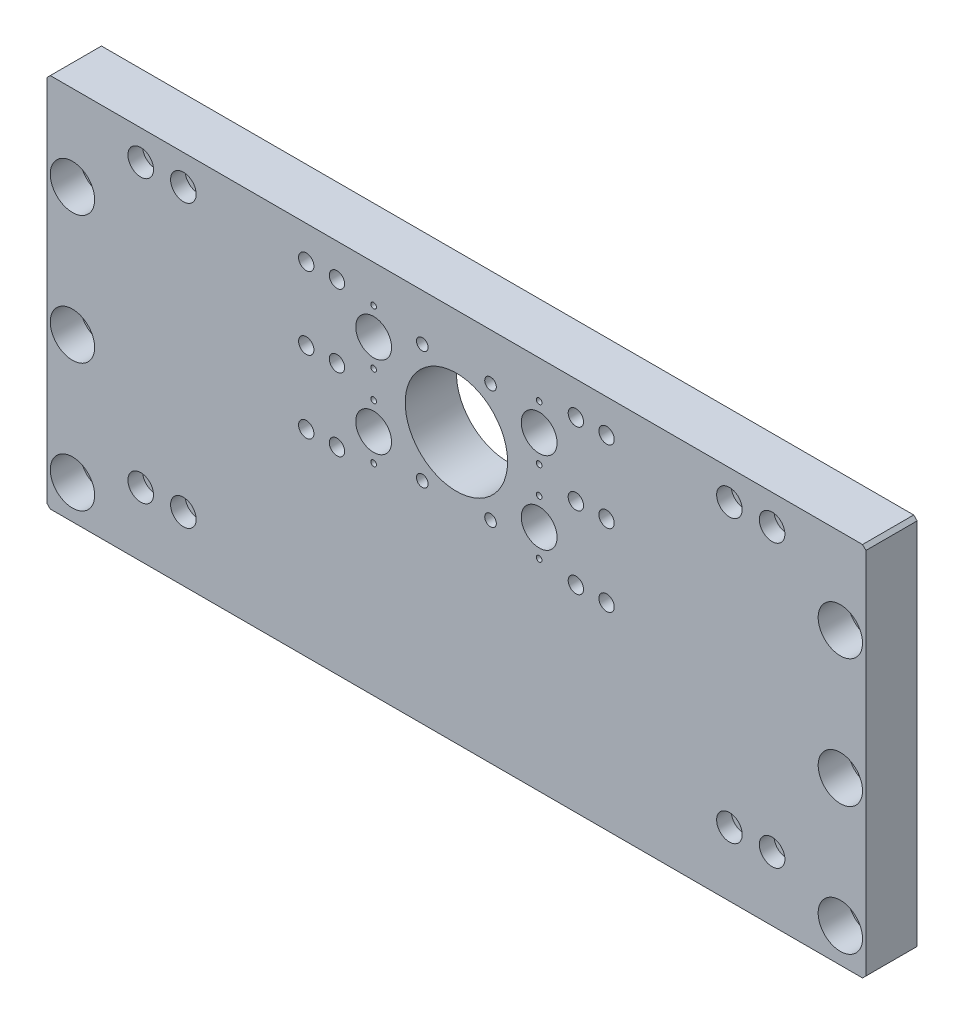
from build123d import *

# Parameters (mm, degrees)
SKETCH1_W                                            = 480
SKETCH1_H                                            = 220
BOSS_EXTRUDE1_DEPTH                                  = 15
HOLE_SIZE_PER_SOCKET_HEAD_CAP_SCREW_TYPE_D           = 17.5
HOLE_SIZE_PER_SOCKET_HEAD_CAP_SCREW_TYPE_CBORE_D     = 26
HOLE_SIZE_PER_SOCKET_HEAD_CAP_SCREW_TYPE_CBORE_DEPTH = 17.5
CHAMFER1_SIZE                                        = 2
SKETCH4_R                                            = 30
CUT_EXTRUDE1_DEPTH                                   = 266.706605112
M8_TAPPED_HOLE1_D                                    = 6.8
M8_TAPPED_HOLE1_DEPTH                                = 19.75
M8_TAPPED_HOLE1_TIP                                  = 2.042926105
HOLE_WIZARD_2_D                                      = 9
HOLE_WIZARD_2_CBORE_D                                = 15
HOLE_WIZARD_2_CBORE_DEPTH                            = 9
SKETCH9_R                                            = 10.5
CUT_EXTRUDE2_DEPTH                                   = 266.706605112
M4_TAPPED_HOLE1_AT_2_COUNT                           = 2
M4_TAPPED_HOLE1_AT_2_PITCH                           = 32
M4_TAPPED_HOLE1_AT_3_COUNT                           = 2
M4_TAPPED_HOLE1_AT_3_PITCH                           = 48
M4_TAPPED_HOLE1_AT_4_COUNT                           = 2
M4_TAPPED_HOLE1_AT_4_PITCH                           = 80
CBORE_FOR_M8_HEX_SOCKET_HEAD_CAP_SCREW1_D            = 9
CBORE_FOR_M8_HEX_SOCKET_HEAD_CAP_SCREW1_CBORE_D      = 15
CBORE_FOR_M8_HEX_SOCKET_HEAD_CAP_SCREW1_CBORE_DEPTH  = 8.6


with BuildPart() as part:
    # Sketch1 → Boss-Extrude1 (new, symmetric)
    with BuildSketch(Plane.XY):
        Rectangle(SKETCH1_W, SKETCH1_H)
    extrude(amount=BOSS_EXTRUDE1_DEPTH, both=True)

    # Hole size per socket head cap screw type2 (through all)
    with Locations(Plane.XY.offset(15)):
        with Locations((-225, 60), (225, 60), (225, -90), (-225, -90), (-225, -15), (225, -15)):
            CounterBoreHole(HOLE_SIZE_PER_SOCKET_HEAD_CAP_SCREW_TYPE_D / 2, HOLE_SIZE_PER_SOCKET_HEAD_CAP_SCREW_TYPE_CBORE_D / 2, HOLE_SIZE_PER_SOCKET_HEAD_CAP_SCREW_TYPE_CBORE_DEPTH)

    # Chamfer1
    chamfer1_edges = [part.edges().sort_by_distance(p)[0] for p in [
        (240, -110, 0),
        (-240, -110, 0),
        (-240, 110, 0),
        (240, 110, 0),
    ]]
    chamfer(chamfer1_edges, length=CHAMFER1_SIZE)

    # Sketch4 → Cut-Extrude1 (cut, through all)
    with BuildSketch(Plane.XY.offset(15)):
        with Locations((0, 48)):
            Circle(SKETCH4_R)
    extrude(amount=-CUT_EXTRUDE1_DEPTH, mode=Mode.SUBTRACT)

    # M8 Tapped Hole1
    with Locations(Plane.XY.offset(15)):
        with Locations((-20, 82.641016151), (20, 82.641016151), (-20, 13.358983849), (20, 13.358983849)):
            Hole(M8_TAPPED_HOLE1_D / 2, depth=M8_TAPPED_HOLE1_DEPTH)
            with Locations((0, 0, -(M8_TAPPED_HOLE1_DEPTH + M8_TAPPED_HOLE1_TIP / 2))):  # 118° drill point
                Cone(0, M8_TAPPED_HOLE1_D / 2, M8_TAPPED_HOLE1_TIP, mode=Mode.SUBTRACT)

    # 打孔尺寸根据内六角圆柱头螺钉的类型2 (through all)
    with Locations(Plane(origin=(0, 0, -15), x_dir=(-1, 0, 0), z_dir=(0, 0, -1))):
        with Locations((-88, 90.5), (-70, 90.5), (-70, 48), (-88, 48), (-88, 5.5), (-70, 5.5), (70, 90.5), (88, 90.5), (70, 48), (88, 48), (70, 5.5), (88, 5.5)):
            CounterBoreHole(HOLE_WIZARD_2_D / 2, HOLE_WIZARD_2_CBORE_D / 2, HOLE_WIZARD_2_CBORE_DEPTH)

    # Sketch9 → Cut-Extrude2 (cut, through all)
    with BuildSketch(Plane.XY.offset(15)):
        with Locations((-48.5, 72)):
            Circle(SKETCH9_R)
        with Locations((-48.5, 24)):
            Circle(SKETCH9_R)
        with Locations((48.5, 24)):
            Circle(SKETCH9_R)
        with Locations((48.5, 72)):
            Circle(SKETCH9_R)
    extrude(amount=-CUT_EXTRUDE2_DEPTH, mode=Mode.SUBTRACT)

    # Sketch10 → M4 Tapped Hole1 (revolve, cut)
    with BuildSketch(Plane(origin=(48.5, 88, 15), x_dir=(0, -1, 0), z_dir=(1, 0, 0))):
        Polygon((0, 0), (0, 11.091420021), (1.65, 10.1), (1.65, 0), align=None)
    m4_tapped_hole1 = revolve(axis=Axis((48.5, 88, 21.35), (0, 0, -1)), mode=Mode.SUBTRACT)

    # M4 Tapped Hole1 at 2: M4 Tapped Hole1 ×2
    with Locations(*[(0, -i * M4_TAPPED_HOLE1_AT_2_PITCH, 0) for i in range(1, M4_TAPPED_HOLE1_AT_2_COUNT)]):
        add(m4_tapped_hole1, mode=Mode.SUBTRACT)

    # M4 Tapped Hole1 at 3: M4 Tapped Hole1 ×2
    with Locations(*[(0, -i * M4_TAPPED_HOLE1_AT_3_PITCH, 0) for i in range(1, M4_TAPPED_HOLE1_AT_3_COUNT)]):
        add(m4_tapped_hole1, mode=Mode.SUBTRACT)

    # M4 Tapped Hole1 at 4: M4 Tapped Hole1 ×2
    with Locations(*[(0, -i * M4_TAPPED_HOLE1_AT_4_PITCH, 0) for i in range(1, M4_TAPPED_HOLE1_AT_4_COUNT)]):
        add(m4_tapped_hole1, mode=Mode.SUBTRACT)

    # Mirror1: M4 Tapped Hole1 across plane
    add(m4_tapped_hole1.mirror(Plane(origin=(0, 0, 0), x_dir=(0, 0, 1), z_dir=(1, 0, 0))), mode=Mode.SUBTRACT)

    # Mirror1 copy 1 sketch → Mirror1 copy 1 (revolve, cut)
    with BuildSketch(Plane(origin=(-48.5, 56, 15), x_dir=(0, -1, 0), z_dir=(-1, 0, 0))):
        Polygon((0, 0), (0, -11.091420021), (1.65, -10.1), (1.65, 0), align=None)
    revolve(axis=Axis((-48.5, 56, 21.35), (0, 0, 1)), mode=Mode.SUBTRACT)

    # Mirror1 copy 2 sketch → Mirror1 copy 2 (revolve, cut)
    with BuildSketch(Plane(origin=(-48.5, 40, 15), x_dir=(0, -1, 0), z_dir=(-1, 0, 0))):
        Polygon((0, 0), (0, -11.091420021), (1.65, -10.1), (1.65, 0), align=None)
    revolve(axis=Axis((-48.5, 40, 21.35), (0, 0, 1)), mode=Mode.SUBTRACT)

    # Mirror1 copy 3 sketch → Mirror1 copy 3 (revolve, cut)
    with BuildSketch(Plane(origin=(-48.5, 8, 15), x_dir=(0, -1, 0), z_dir=(-1, 0, 0))):
        Polygon((0, 0), (0, -11.091420021), (1.65, -10.1), (1.65, 0), align=None)
    revolve(axis=Axis((-48.5, 8, 21.35), (0, 0, 1)), mode=Mode.SUBTRACT)

    # CBORE for M8 Hex Socket Head Cap Screw1 (through all)
    with Locations(Plane.XY.offset(15)):
        with Locations((-185, -72.5), (-160, -72.5), (-185, 92.5), (-160, 92.5), (185, 92.5), (160, 92.5), (185, -72.5), (160, -72.5)):
            CounterBoreHole(CBORE_FOR_M8_HEX_SOCKET_HEAD_CAP_SCREW1_D / 2, CBORE_FOR_M8_HEX_SOCKET_HEAD_CAP_SCREW1_CBORE_D / 2, CBORE_FOR_M8_HEX_SOCKET_HEAD_CAP_SCREW1_CBORE_DEPTH)


solid = part.part
